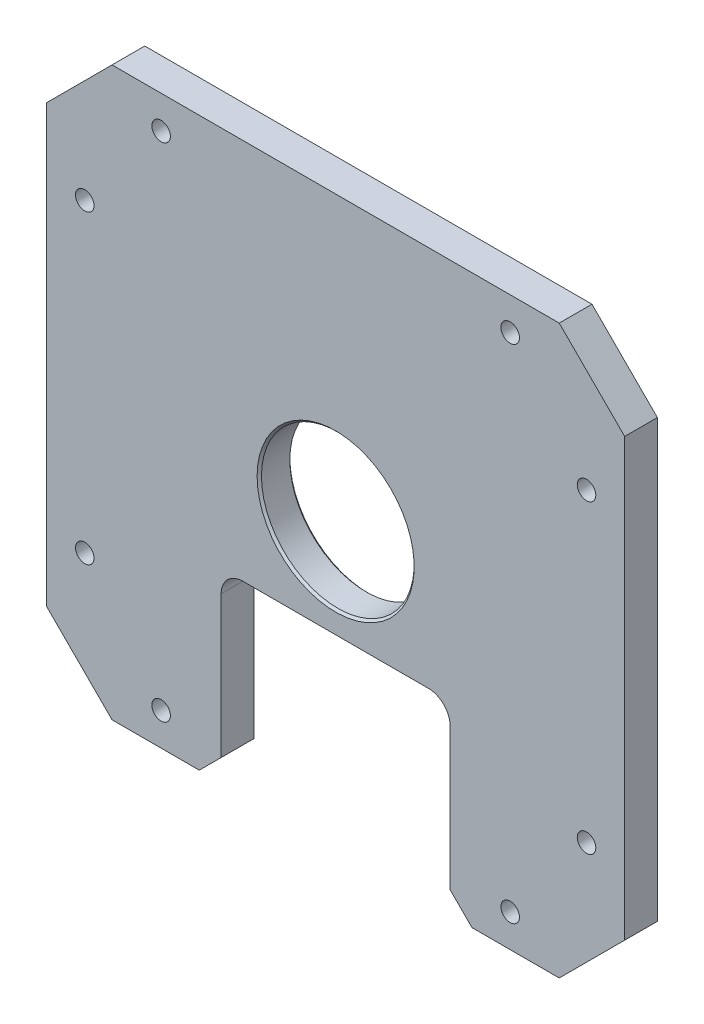
from build123d import *

# Parameters (mm, degrees)
SKETCH_1_W          = 265
SKETCH_1_H          = 260
EXTRUDE_1_DEPTH     = 15
HOLE_WIZARD_M10_1_D = 8.5
SKETCH_4_W          = 105
SKETCH_4_H          = 85
CUT_EXTRUDE_1_DEPTH = 187.229025665
FILLET_1_R          = 10
SKETCH_5_R          = 35
CUT_EXTRUDE_2_DEPTH = 187.229025665
CHAMFER_2_SIZE      = 1
CHAMFER_1_SIZE      = 30
CHAMFER_3_SIZE      = 10


with BuildPart() as part:
    # 草图1 → 凸台-拉伸1 (new body)
    with BuildSketch(Plane.XY):
        Rectangle(SKETCH_1_W, SKETCH_1_H)
    extrude(amount=EXTRUDE_1_DEPTH)

    # M10 螺纹孔1 (through all)
    with Locations(Plane(origin=(0, 0, 0), x_dir=(-1, 0, 0), z_dir=(0, 0, -1))):
        with Locations((-80, 115), (-115, 70), (-115, -70), (-80, -115), (80, -115), (115, -70), (115, 70), (80, 115)):
            Hole(HOLE_WIZARD_M10_1_D / 2)

    # 草图4 → 切除-拉伸1 (cut, through all)
    with BuildSketch(Plane(origin=(0, 0, 0), x_dir=(-1, 0, 0), z_dir=(0, 0, -1))):
        with Locations((0, -87.5)):
            Rectangle(SKETCH_4_W, SKETCH_4_H)
    extrude(amount=-CUT_EXTRUDE_1_DEPTH, mode=Mode.SUBTRACT)

    # 圆角1
    fillet_1_edges = [part.edges().sort_by_distance(p)[0] for p in [
        (52.5, -45, 7.5),
        (-52.5, -45, 7.5),
    ]]
    fillet(fillet_1_edges, radius=FILLET_1_R)

    # 草图5 → 切除-拉伸2 (cut, through all)
    with BuildSketch(Plane(origin=(0, 0, 0), x_dir=(-1, 0, 0), z_dir=(0, 0, -1))):
        Circle(SKETCH_5_R)
    extrude(amount=-CUT_EXTRUDE_2_DEPTH, mode=Mode.SUBTRACT)

    # 倒角2
    chamfer_2_edges = [part.edges().sort_by_distance(p)[0] for p in [
        (35, 0, 15),
        (35, 0, 0),
    ]]
    chamfer(chamfer_2_edges, length=CHAMFER_2_SIZE)

    # 倒角1
    chamfer_1_edges = [part.edges().sort_by_distance(p)[0] for p in [
        (132.5, -130, 7.5),
        (-132.5, -130, 7.5),
        (-132.5, 130, 7.5),
        (132.5, 130, 7.5),
    ]]
    chamfer(chamfer_1_edges, length=CHAMFER_1_SIZE)

    # 倒角3
    chamfer_3_edges = [part.edges().sort_by_distance(p)[0] for p in [
        (52.5, -130, 7.5),
        (-52.5, -130, 7.5),
    ]]
    chamfer(chamfer_3_edges, length=CHAMFER_3_SIZE)


solid = part.part
